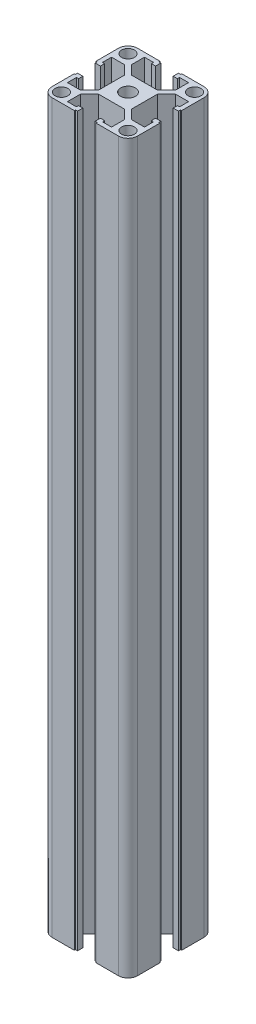
SolidWorks part; units mm, degrees
ref_plane "主视基准图" through (0, 0, 0) normal (0, 0, 1) x (1, 0, 0)
ref_plane "上视基准图" through (0, 0, 0) normal (0, 1, 0) x (1, 0, 0)
ref_plane "右视基准图" through (0, 0, 0) normal (1, 0, 0) x (0, 0, -1)
sketch "草图1" plane through (0, 0, 0) normal (0, 0, 1) x (1, 0, 0)
  line L0 (0, 0) -> (0, 340)
  dimension "D1" = 340
other "结构构件1"
ref_plane "基准面1" through (0, 0, 0) normal (0, 1, 0) x (-1, 0, 0)
sketch "Sketch16" plane through (0, 0, 0) normal (0, 1, 0) x (-1, 0, 0)
  line L0 (-5.1, 20) -> (-5.1, 19.5)
  line L1 (-5.1, 19.5) -> (-4.1, 19.5)
  line L2 (-4.1, 19.5) -> (-4.1, 17)
  line L3 (-6.1, 18) -> (-10.3, 18)
  line L4 (-15.5, -20) -> (-5.1, -20)
  line L5 (-20, -15.5) -> (-20, -5.1)
  line L6 (15.5, 20) -> (5.1, 20)
  line L7 (20, 15.5) -> (20, 5.1)
  line L8 (0, 14.8756) -> (0, 0) construction
  line L9 (0, 0) -> (14.1675, 0) construction
  line L10 (-10.3, 18) -> (-10.3, 12)
  line L11 (-10.3, 12) -> (-6, 7.7)
  line L12 (-6, 7.7) -> (6, 7.7)
  line L13 (10.3, 12) -> (6, 7.7)
  line L14 (10.3, 18) -> (10.3, 12)
  line L15 (6.1, 18) -> (10.3, 18)
  line L16 (4.1, 19.5) -> (4.1, 17)
  line L17 (5.1, 19.5) -> (4.1, 19.5)
  line L18 (5.1, 20) -> (5.1, 19.5)
  line L19 (-5.1, 20) -> (-15.5, 20)
  line L20 (20, 5.1) -> (19.5, 5.1)
  line L21 (0, 0) -> (-15.5563, 15.5563) construction
  line L22 (0, 0) -> (-15.5563, -15.5563) construction
  line L25 (19.5, 5.1) -> (19.5, 4.1)
  line L26 (19.5, 4.1) -> (17, 4.1)
  line L27 (17, 6.1) -> (17, 4.1)
  line L28 (18, 6.1) -> (17, 6.1)
  line L29 (18, 6.1) -> (18, 10.3)
  line L30 (18, 10.3) -> (12, 10.3)
  line L31 (12, 10.3) -> (7.7, 6)
  line L32 (7.7, 6) -> (7.7, -6)
  line L33 (12, -10.3) -> (7.7, -6)
  line L34 (18, -10.3) -> (12, -10.3)
  line L35 (18, -6.1) -> (18, -10.3)
  line L36 (18, -6.1) -> (17, -6.1)
  line L37 (17, -4.1) -> (17, -6.1)
  line L38 (19.5, -4.1) -> (17, -4.1)
  line L39 (19.5, -5.1) -> (19.5, -4.1)
  line L40 (20, -5.1) -> (19.5, -5.1)
  line L41 (5.1, -20) -> (5.1, -19.5)
  line L42 (5.1, -19.5) -> (4.1, -19.5)
  line L43 (4.1, -19.5) -> (4.1, -17)
  line L44 (6.1, -17) -> (4.1, -17)
  line L45 (6.1, -18) -> (6.1, -17)
  line L46 (6.1, -18) -> (10.3, -18)
  line L47 (10.3, -18) -> (10.3, -12)
  line L48 (10.3, -12) -> (6, -7.7)
  line L49 (6, -7.7) -> (-6, -7.7)
  line L50 (-10.3, -12) -> (-6, -7.7)
  line L51 (-10.3, -18) -> (-10.3, -12)
  line L52 (-6.1, -18) -> (-10.3, -18)
  line L53 (-6.1, -18) -> (-6.1, -17)
  line L54 (-4.1, -17) -> (-6.1, -17)
  line L55 (-4.1, -19.5) -> (-4.1, -17)
  line L56 (-5.1, -19.5) -> (-4.1, -19.5)
  line L57 (-5.1, -20) -> (-5.1, -19.5)
  line L58 (-20, -5.1) -> (-19.5, -5.1)
  line L59 (5.1, -20) -> (15.5, -20)
  line L60 (-20, 5.1) -> (-20, 15.5)
  line L61 (-19.5, -5.1) -> (-19.5, -4.1)
  line L62 (-6.1, 18) -> (-6.1, 17)
  line L63 (-6.1, 17) -> (-4.1, 17)
  line L64 (6.1, 18) -> (6.1, 17)
  line L65 (4.1, 17) -> (6.1, 17)
  line L66 (-19.5, -4.1) -> (-17, -4.1)
  line L71 (-17, -6.1) -> (-17, -4.1)
  line L72 (-18, -6.1) -> (-17, -6.1)
  line L73 (-18, -6.1) -> (-18, -10.3)
  line L74 (-18, -10.3) -> (-12, -10.3)
  line L75 (-12, -10.3) -> (-7.7, -6)
  line L76 (-7.7, -6) -> (-7.7, 6)
  line L77 (-12, 10.3) -> (-7.7, 6)
  line L78 (-18, 10.3) -> (-12, 10.3)
  line L79 (-18, 6.1) -> (-18, 10.3)
  line L80 (-18, 6.1) -> (-17, 6.1)
  line L81 (-17, 4.1) -> (-17, 6.1)
  line L82 (-19.5, 4.1) -> (-17, 4.1)
  line L83 (-19.5, 5.1) -> (-19.5, 4.1)
  line L84 (-20, 5.1) -> (-19.5, 5.1)
  line L85 (20, -5.1) -> (20, -15.5)
  circle A0 centre (0, 0) radius 3.4
  arc A1 (-20, 15.5) -> (-15.5, 20) centre (-15.5, 15.5) cw
  arc A2 (20, 15.5) -> (15.5, 20) centre (15.5, 15.5) ccw
  arc A3 (-15.5, -20) -> (-20, -15.5) centre (-15.5, -15.5) cw
  arc A4 (15.5, -20) -> (20, -15.5) centre (15.5, -15.5) ccw
  circle A5 centre (-15.5563, 15.5563) radius 3
  circle A6 centre (15.5563, 15.5563) radius 3
  circle A7 centre (15.5563, -15.5563) radius 3
  circle A8 centre (-15.5563, -15.5563) radius 3
  point P2 (0, 10)
  point P3 (0, 0)
  point P4 (0, 0)
  point P5 (-20, -20)
  point P6 (20, -20)
  point P7 (20, 20)
  point P8 (-20, 20)
  point P36 (-20, 20)
  point P39 (20, 20)
  dimension "D1" = 20.6
  dimension "D2" = 40
  dimension "D3" = 8.2
  dimension "D4" = 10.2
  dimension "D5" = 12.3
  dimension "D6" = 6.8
  dimension "D7" = 4.5
  dimension "D8" = 45
  dimension "D12" = 6
  dimension "D13" = 22
  dimension "D9" = 0.5
  dimension "D10" = 2
  dimension "D11" = 12
  dimension "D16" = 3
  dimension "D17" = 2
hole_wizard "M8 螺纹孔3" positions "草图7" profile "草图6" tap size "M8" standard "Gb"
sketch "草图7" plane through (0, 340, 0) normal (0, 1, 0) x (1, 0, 0)
  circle A0 centre (0, 0) radius 3.4 construction
  point P0 (0, 0)
sketch "草图6" plane through (0, 340, 0) normal (1, 0, 0) x (0, 0, 1)
  line L0 (0, 0) -> (0, 21.823)
  line L1 (0, 21.823) -> (3.45, 19.75)
  line L2 (3.45, 19.75) -> (3.45, 0)
  line L5 (3.45, 0) -> (0, 0)
  line L10 (0, 21.823) -> (-3.45, 19.75) construction
  line L11 (0, -6.35) -> (0, 107.95) construction
  dimension "螺纹孔钻头直径" = 6.9
  dimension "螺纹孔钻头深度" = 19.75
  dimension "导头角度" = 118
cosmetic thread "孔螺蚊线1" parameters "D1"=16, "D2"=8
